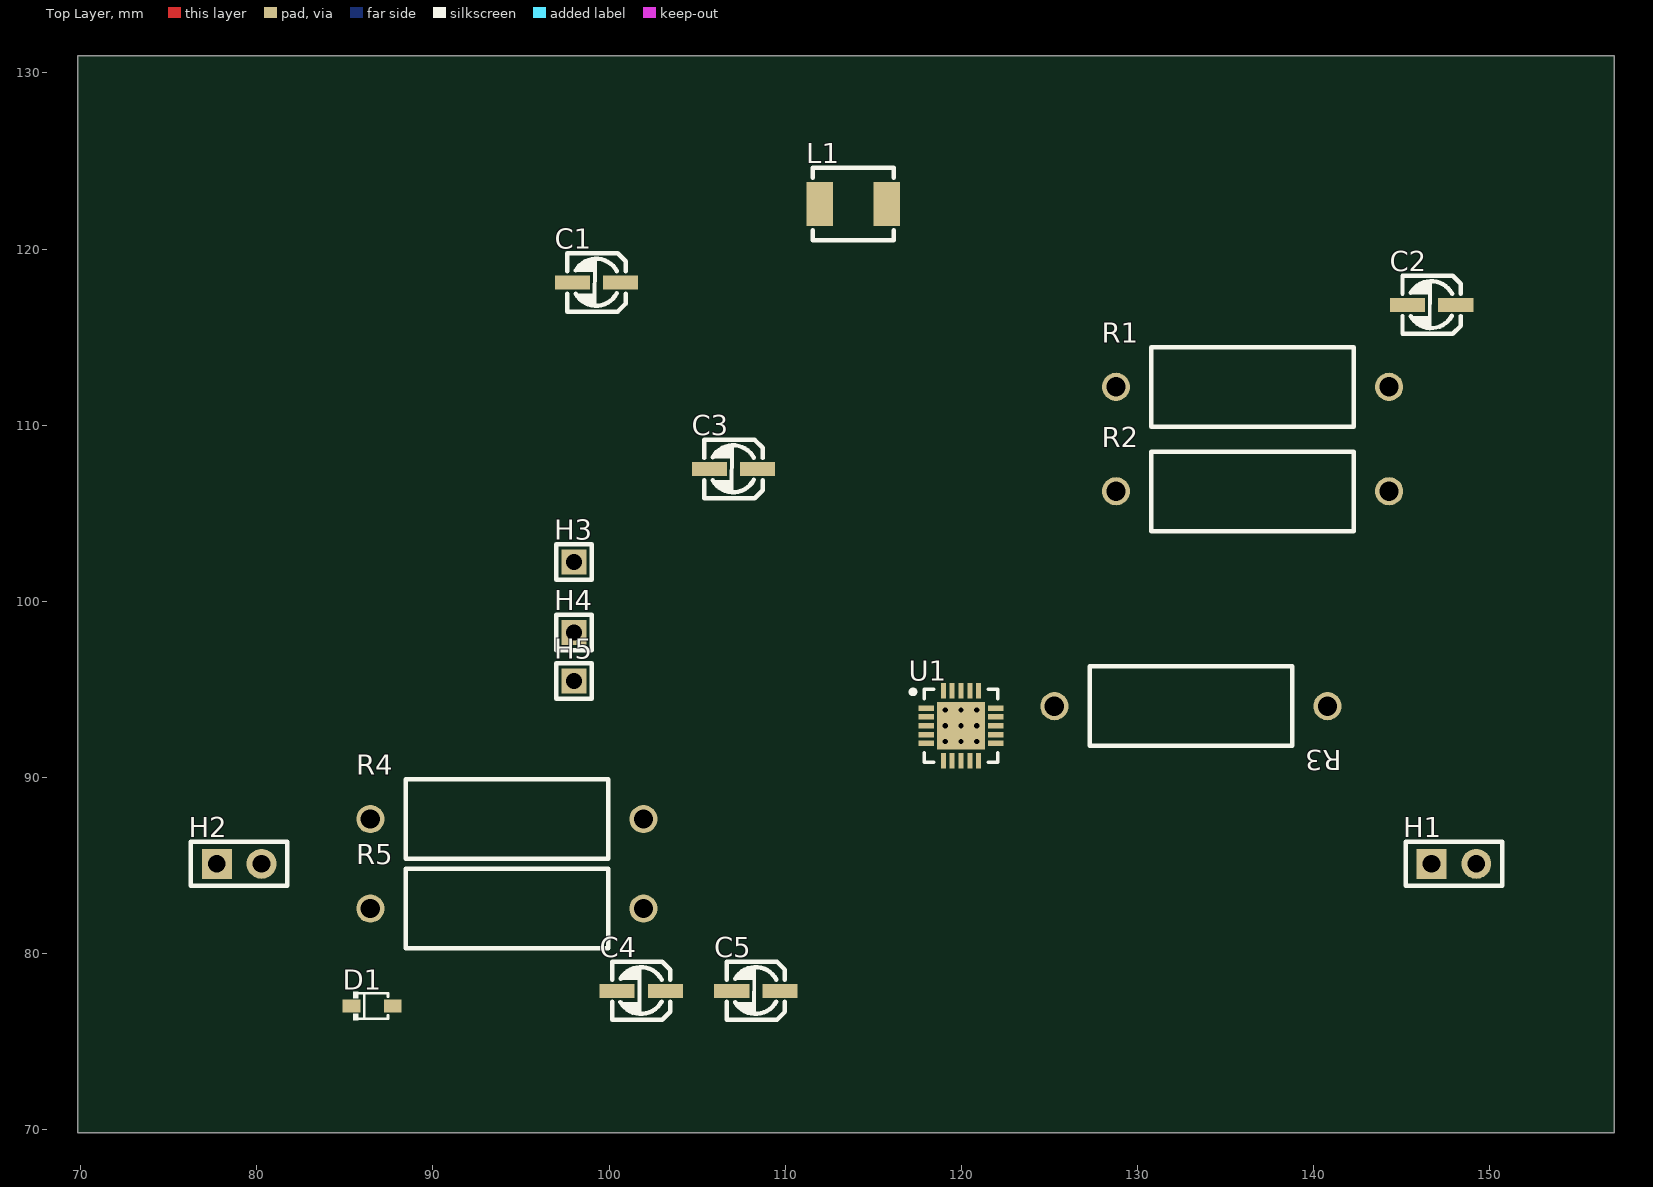
[diagram p0: Top Layer view]
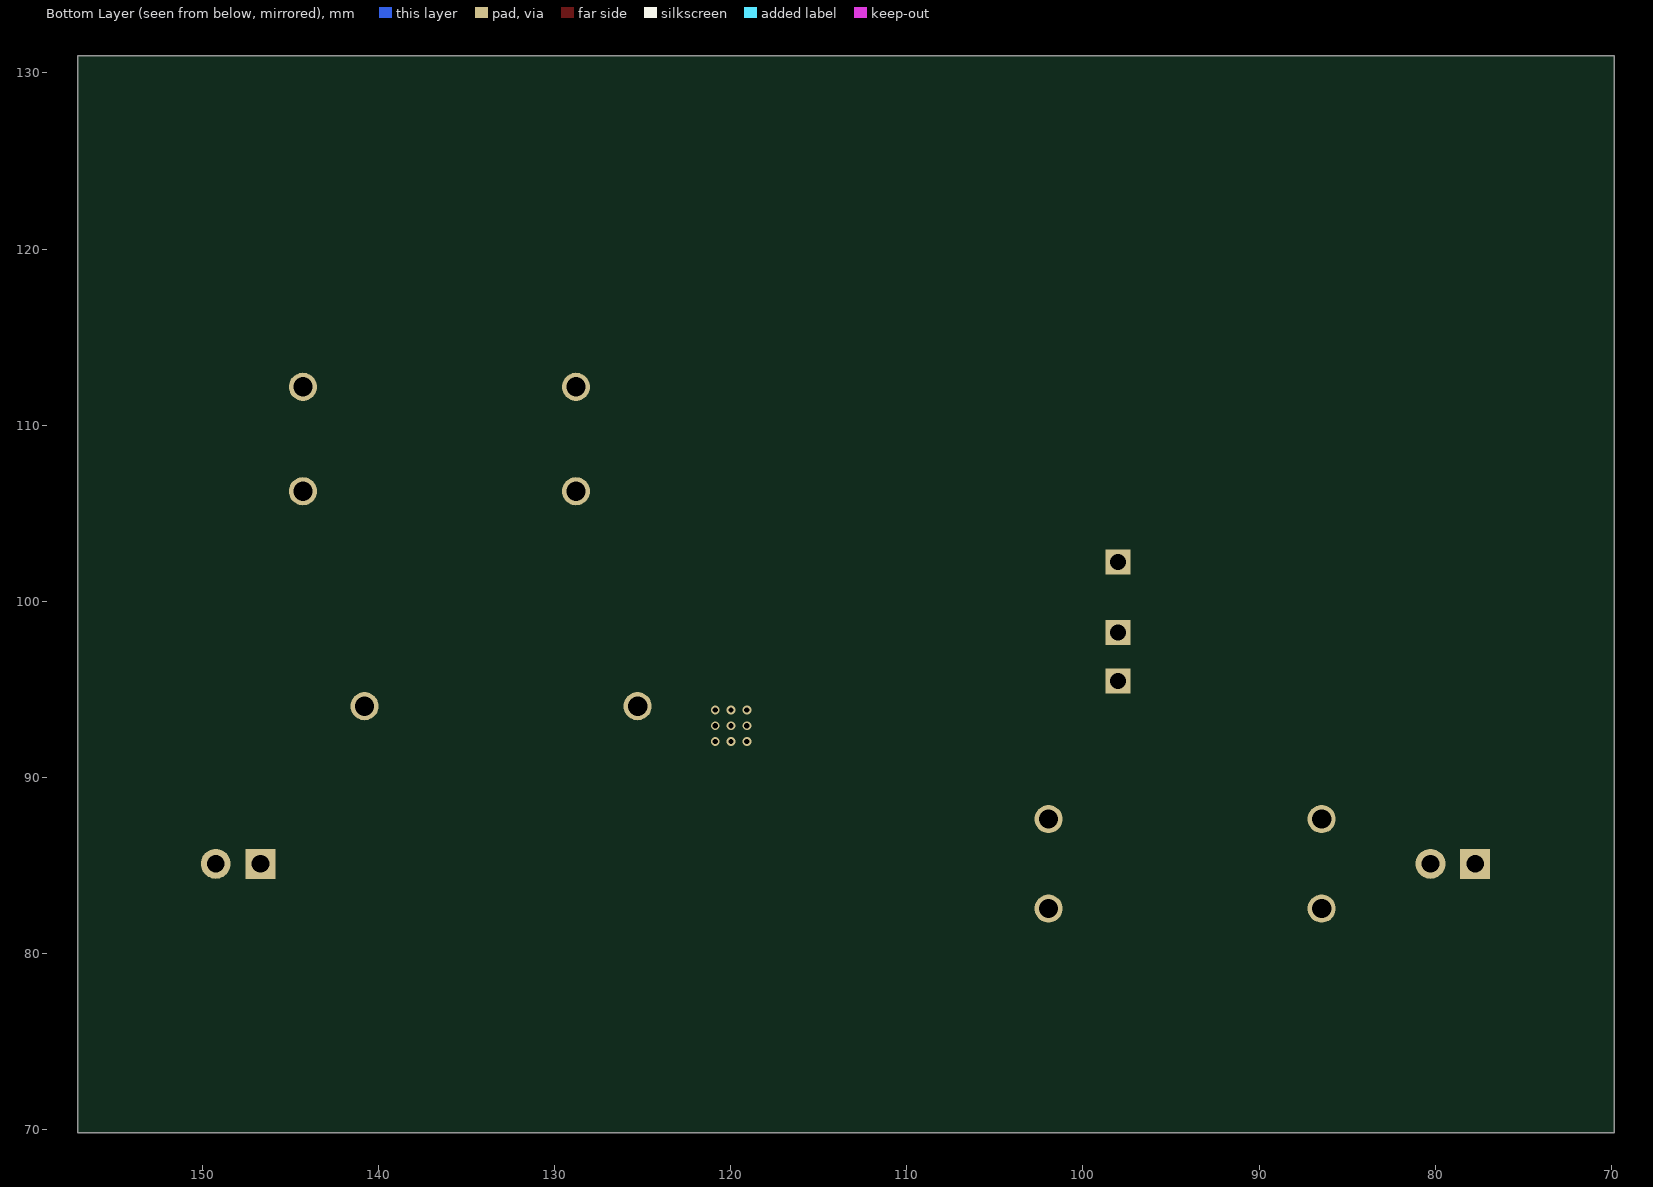
[diagram p1: Bottom Layer view, seen from below]
# Altium PCB MISC50934.pcbdoc
Units mm, origin at the board's own origin, x right, y up, seen from the top; angles counter-clockwise.
Board outline 87.19 x 61.12 mm, 2 copper layers (Top Layer, Bottom Layer), stack 0.07 mm thick; 18 components, 16 nets, 52 pads, 9 vias.

## Layer stack, top to bottom
Top Solder Mask Layer: solder mask 0.01, Dk 3.3
Top Layer: signal copper 0.035
Bottom Layer: signal copper 0.035
Bottom Solder Mask Layer: solder mask 0.01, Dk 3.3

## Board outline
157.044,69.85 69.85,69.85 69.85,130.966 157.044,130.966

## Design rules (kind name [scope] priority, off if disabled: settings)
BoardOutlineClearance Plane_innerPlane_1 [All] p2 off: genericclearance=0.102 ignorepadtopadclearanceinfootprint=FALSE except(0: Arc-SplitContinuation Track-SplitContinuation SMDPad-SplitContinuation THPad-SplitContinuation Via-SplitContinuation Fill-SplitContinuation Region-SplitContinuation Poly-SplitContinuation Text-SplitContinuation Hole-SplitContinuation; 0.152: Arc-CutoutEdge Track-CutoutEdge SMDPad-CutoutEdge THPad-CutoutEdge Via-CutoutEdge Text-CutoutEdge; 0.175: Hole-OutlineEdge Hole-CutoutEdge; 0.254: Poly-OutlineEdge Poly-CutoutEdge; 0.3: Arc-OutlineEdge Track-OutlineEdge SMDPad-OutlineEdge THPad-OutlineEdge Via-OutlineEdge Fill-OutlineEdge Region-OutlineEdge Text-OutlineEdge Fill-CutoutEdge Region-CutoutEdge)
BoardOutlineClearance Copper_copperRegion_1 [All] p4 off: genericclearance=0.102 ignorepadtopadclearanceinfootprint=FALSE except(0: Arc-SplitContinuation Track-SplitContinuation SMDPad-SplitContinuation THPad-SplitContinuation Via-SplitContinuation Fill-SplitContinuation Region-SplitContinuation Poly-SplitContinuation Text-SplitContinuation Hole-SplitContinuation; 0.152: Arc-CutoutEdge Track-CutoutEdge SMDPad-CutoutEdge THPad-CutoutEdge Via-CutoutEdge Text-CutoutEdge; 0.175: Hole-OutlineEdge Hole-CutoutEdge; 0.254: Poly-OutlineEdge Poly-CutoutEdge; 0.3: Arc-OutlineEdge Track-OutlineEdge SMDPad-OutlineEdge THPad-OutlineEdge Via-OutlineEdge Fill-OutlineEdge Region-OutlineEdge Text-OutlineEdge Fill-CutoutEdge Region-CutoutEdge)
BoardOutlineClearance copperThickness1oz_1 [All] p6: genericclearance=0.102 ignorepadtopadclearanceinfootprint=FALSE except(0: Arc-SplitContinuation Track-SplitContinuation SMDPad-SplitContinuation THPad-SplitContinuation Via-SplitContinuation Fill-SplitContinuation Region-SplitContinuation Poly-SplitContinuation Text-SplitContinuation Hole-SplitContinuation; 0.152: Arc-CutoutEdge Track-CutoutEdge SMDPad-CutoutEdge THPad-CutoutEdge Via-CutoutEdge Text-CutoutEdge; 0.175: Hole-OutlineEdge Hole-CutoutEdge; 0.254: Poly-OutlineEdge Poly-CutoutEdge; 0.3: Arc-OutlineEdge Track-OutlineEdge SMDPad-OutlineEdge THPad-OutlineEdge Via-OutlineEdge Fill-OutlineEdge Region-OutlineEdge Text-OutlineEdge Fill-CutoutEdge Region-CutoutEdge)
Clearance Plane_innerPlane [All] p1 off: gap=0.102 ignorepadtopadclearanceinfootprint=FALSE except(0.152: SMDPad-Track SMDPad-SMDPad THPad-Track SMDPad-THPad THPad-THPad Track-Via SMDPad-Via THPad-Via Via-Via Fill-SMDPad Region-SMDPad Fill-THPad Region-THPad Fill-Via Region-Via Fill-Fill Fill-Region Region-Region Arc-Track Arc-SMDPad Arc-THPad Arc-Via Fill-Arc Region-Arc Arc-Arc Text-Track SMDPad-Text Text-THPad Text-Via Fill-Text Region-Text Arc-Text Text-Text; 0.175: Hole-Track Hole-SMDPad Hole-THPad Hole-Via Fill-Hole Region-Hole Hole-Arc Hole-Text; 0.254: Poly-Track Poly-SMDPad Poly-THPad Poly-Via Poly-Fill Poly-Region Poly-Poly Poly-Arc Poly-Text Poly-Hole; 0.3: Fill-Track Region-Track)
Clearance Copper_copperRegion [All] p3 off: gap=0.102 ignorepadtopadclearanceinfootprint=FALSE except(0.152: SMDPad-Track SMDPad-SMDPad THPad-Track SMDPad-THPad THPad-THPad Track-Via SMDPad-Via THPad-Via Via-Via Fill-SMDPad Region-SMDPad Fill-THPad Region-THPad Fill-Via Region-Via Fill-Fill Fill-Region Region-Region Arc-Track Arc-SMDPad Arc-THPad Arc-Via Fill-Arc Region-Arc Arc-Arc Text-Track SMDPad-Text Text-THPad Text-Via Fill-Text Region-Text Arc-Text Text-Text; 0.175: Hole-Track Hole-SMDPad Hole-THPad Hole-Via Fill-Hole Region-Hole Hole-Arc Hole-Text; 0.254: Poly-Track Poly-SMDPad Poly-THPad Poly-Via Poly-Fill Poly-Region Poly-Poly Poly-Arc Poly-Text Poly-Hole; 0.3: Fill-Track Region-Track)
Clearance copperThickness1oz [All] p5: gap=0.102 ignorepadtopadclearanceinfootprint=FALSE except(0.152: SMDPad-Track SMDPad-SMDPad THPad-Track SMDPad-THPad THPad-THPad Track-Via SMDPad-Via THPad-Via Via-Via Fill-SMDPad Region-SMDPad Fill-THPad Region-THPad Fill-Via Region-Via Fill-Fill Fill-Region Region-Region Arc-Track Arc-SMDPad Arc-THPad Arc-Via Fill-Arc Region-Arc Arc-Arc Text-Track SMDPad-Text Text-THPad Text-Via Fill-Text Region-Text Arc-Text Text-Text; 0.175: Hole-Track Hole-SMDPad Hole-THPad Hole-Via Fill-Hole Region-Hole Hole-Arc Hole-Text; 0.254: Poly-Track Poly-SMDPad Poly-THPad Poly-Via Poly-Fill Poly-Region Poly-Poly Poly-Arc Poly-Text Poly-Hole; 0.3: Fill-Track Region-Track)
DiffPairsRouting differentialPair [All] p1: maxlimit=0.152 minlimit=0.127 mostfreqgap=0.152 toplayer_minwidth=0.127 toplayer_prefwidth=2.54 toplayer_maxwidth=2.54 toplayer_mingap=0.127 toplayer_prefgap=0.152 toplayer_maxgap=0.152 bottomlayer_minwidth=0.127 bottomlayer_prefwidth=2.54 bottomlayer_maxwidth=2.54 bottomlayer_mingap=0.127 bottomlayer_prefgap=0.152 bottomlayer_maxgap=0.152 maxuncoupledlength=0.254
HoleToHoleClearance otherClearance [All] p1: gap=0.3 allowstackedmicrovias=TRUE
Length netLength [All] p1: minlimit=0 maxlimit=0
PasteMaskExpansion pasteMaskExpansion [All] p1: expansion=0
PlaneConnect innerPlane [All] p1: planeconnectstyle=Relief reliefexpansion=0.508 reliefentries=4 reliefconductorwidth=0.254 reliefairgap=0.254
PolygonConnect copperRegion [All] p1: connectstyle=Relief reliefconductorwidth=0.254 reliefentries=4 polygonreliefangle="90 Angle" airgapwidth=0.254 via.connectstyle=Relief via.reliefconductorwidth=0.254 via.reliefentries=4 via.polygonreliefangle="90 Angle" via.airgapwidth=0.254
RoutingVias viaSize [All] p1: holewidth=0.61 width=0.305 viastyle="Through Hole" minholewidth=0.5 minwidth=0.3 maxholewidth=10 maxwidth=6.299
SolderMaskExpansion solderMaskExpansion [IsVia] p1: expansion=-25.4 istentingtop=TRUE
SolderMaskExpansion solderMaskExpansion [All] p2: expansion=0.051 istentingtop=FALSE
Width copperThickness1oz_2 [All] p1: maxlimit=2.54 minlimit=0.127 preferedwidth=0.254

## Components (designator, comment, footprint, x,y, rotation, side; value= is the part's Value field where it differs from the comment)
C1 "0.1uF" C_Ele_SMD_3x5.4mm 99.279,118.119 r0 top
C2 "100nF/250V" C_Ele_SMD_3x5.4mm 146.684,116.849 r0 top
C3 "0.1u" C_Ele_SMD_3x5.4mm 107.057,107.529 r0 top
C4 "10nF" C_Ele_SMD_3x5.4mm 101.819,77.913 r0 top
C5 "10nF" C_Ele_SMD_3x5.4mm 108.327,77.913 r0 top
D1 "BAT165E6327" SOD-323_L1.8-W1.3-LS2.5-RD 86.547,77.038 r0 top
H1 "" HDR-TH_2P-P2.54-V-F 147.954,85.11 r0 top
H2 "" HDR-TH_2P-P2.54-V-F 79,85.11 r0 top
H3 "" HDR-TH_1P-V-M_XKB_X4611WV-01I-C28D40 98.009,102.244 r0 top
H4 "" HDR-TH_1P-V-M_XKB_X4611WV-01I-C28D40 98.009,98.24 r0 top
H5 "" HDR-TH_1P-V-M_XKB_X4611WV-01I-C28D40 98.009,95.486 r0 top
L1 "4.7uH" IND-SMD_L4.6-W4.1-A 113.85,122.566 r0 top
R1 "1.72M" Res_1W 136.524,112.186 r0 top
R2 "15k" Res_1W 136.524,106.259 r0 top
R3 "18k" Res_1W 133.029,94.056 r180 top
R4 "1k" Res_1W 94.199,87.65 r0 top
R5 "1k" Res_1W 94.199,82.57 r0 top
U1 "DRV2700" TI-RGP20-2700X2700TP_V 119.974,92.946 r0 top

## Footprints (in the part's own frame and the unit in brackets; to place one, negate y for a bottom-side part, rotate by r counter-clockwise, add the part's x,y. Pads: shape width x height; smd on the part's side, far side on the other; paste and mask are expansions set on the pad)
C_Ele_SMD_3x5.4mm [mil]
  rect 78.7x31.5 smd paste+0 mask+2: 1(54.1,-0.55) 2(-53.7,-0.55)
  silkscreen extent -65,-65 65,65
HDR-TH_1P-V-M_XKB_X4611WV-01I-C28D40 [mm]
  rect 1.4x1.4 hole 0.9: 1(0,0)
  silkscreen extent -1,-1 1,1
HDR-TH_2P-P2.54-V-F [mm]
  rect 1.7x1.7 hole 1: 1(-1.27,0)
  round 1.7 hole 1: 2(1.27,0)
  silkscreen extent -2.74,-1.25 2.74,1.25
IND-SMD_L4.6-W4.1-A [mm]
  rect 1.5x2.5 smd: 1(-1.9,0) 2(1.9,0)
  silkscreen extent -2.3,-2.05 2.3,2.05
Res_1W [mm]
  round 1.6 hole 1.1 paste+0 mask+0.051: 1(-7.75,0) 2(7.75,0)
  silkscreen extent -5.75,-2.26 5.75,2.25
SOD-323_L1.8-W1.3-LS2.5-RD [mm]
  rect 1x0.75 smd: 1(-1.173,0) 2(1.173,0)
  silkscreen extent -1.08,-0.8 0.9,0.8
TI-RGP20-2700X2700TP_V [mil]
  rect 34.5x11.5 smd paste+0 mask+4: 1(-78,39) 2(-78,20) 3(-78,0) 4(-78,-20) 5(-78,-39) 11(78,-39) 12(78,-20) 13(78,0) 14(78,20) 15(78,39)
  rect 11.5x34.5 smd paste+0 mask+4: 6(-39,-78) 7(-20,-78) 8(0,-78) 9(20,-78) 10(39,-78) 16(39,78) 17(20,78) 18(0,78) 19(-20,78) 20(-39,78)
  rect 106.5x106.5 smd paste+0 mask+4: 21(0,0)
  silkscreen extent -112,-82 82,82

## Via types
v1: diameter 0.5, hole 0.3, Top Layer to Bottom Layer, 9 vias

## Nets (pads, with @x,y where several pads share a name; then routed paths per layer and width w, separated by ;. In a path a pad name is that pad's centre, name@x,y a point inside that pad or via, vN(x,y) a via of type N, cw(c..) or ccw(c..) an arc to the next point about the centre after c; other vN are vias at no path point)
$1N1: H1.1 U1.13
$1N2: H1.2 U1.14
$1N6: L1.2 U1.8
$1N7: C2.1 R1.2 U1.10 U1.12
$1N8: R1.1 R2.2 U1.3
$1N11: H3.1 U1.20
$1N12: H4.1 U1.18
$1N13: H5.1 U1.19
$1N14: C3.1 U1.1
$1N16: R3.2 U1.15
$1N18: C4.1 R4.2 U1.17
$1N19: C5.1 R5.2 U1.16
$1N22: D1.1 H2.1 R5.1
$1N23: H2.2 R4.1
GND: C1.2 C2.2 C3.2 C4.2 C5.2 D1.2 R2.1 R3.1 U1.4 U1.5 U1.6 U1.21
  other v1: 119.075,92.047 119.974,92.047 120.874,92.047 119.075,92.946 119.974,92.946 120.874,92.946 119.075,93.845 119.974,93.845 120.874,93.845
VCC: C1.1 L1.1 U1.2
pads on no net: U1.7 U1.9 U1.11